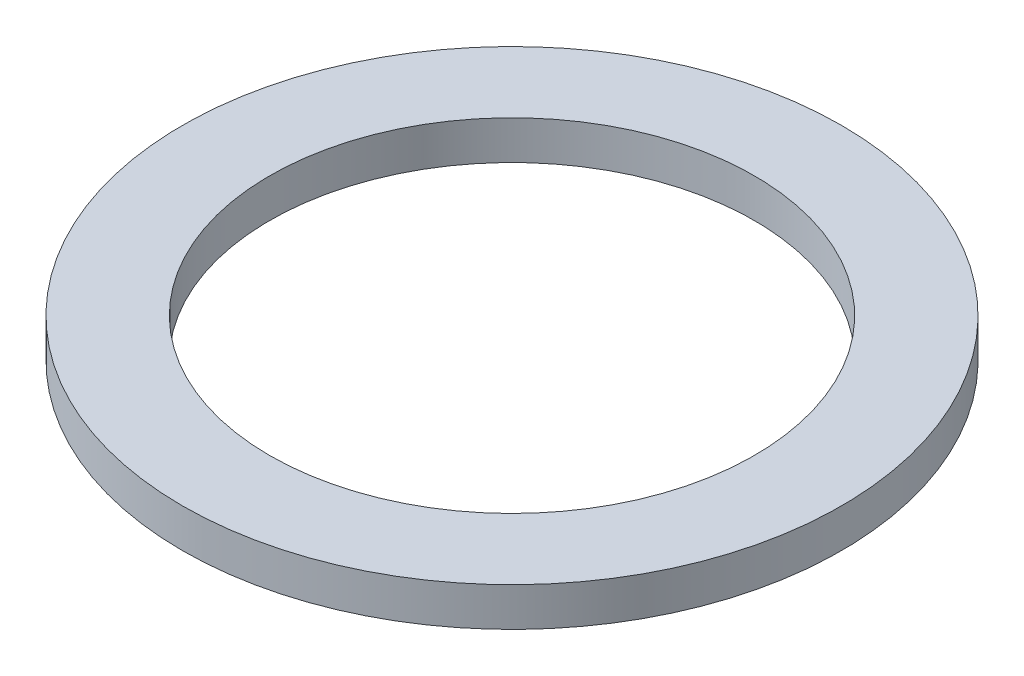
SolidWorks part; units mm, degrees
material "A3"
ref_plane "前视基准面" through (0, 0, 0) normal (0, 0, 1) x (1, 0, 0)
ref_plane "上视基准面" through (0, 0, 0) normal (0, 1, 0) x (1, 0, 0)
ref_plane "右视基准面" through (0, 0, 0) normal (1, 0, 0) x (0, 0, -1)
sketch "草图1" plane through (0, 0, 0) normal (0, 1, 0) x (1, 0, 0)
  circle A0 centre (0, 0) radius 12.5
  circle A1 centre (0, 0) radius 17
  dimension "D1" = 25
  dimension "D2" = 34
extrude "凸台-拉伸1" add sketch "草图1" along normal mid plane 2
